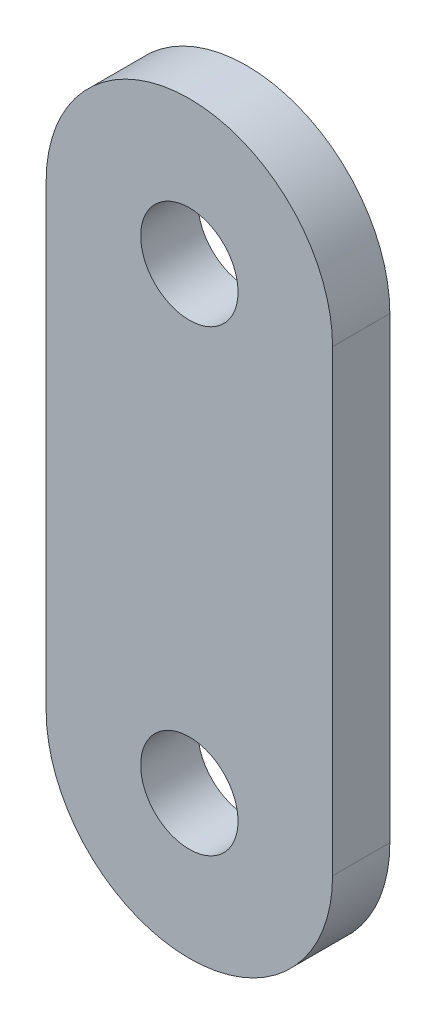
from build123d import *

# Parameters (mm, degrees)
SKETCH1_R           = 8.5
BOSS_EXTRUDE1_DEPTH = 10


with BuildPart() as part:
    # Sketch1 → Boss-Extrude1 (new body)
    with BuildSketch(Plane.XY):
        with BuildLine():
            Line((-25, 0), (-25, 80))
            ThreePointArc((-25, 80), (0, 105), (25, 80))
            Line((25, 80), (25, 0))
            ThreePointArc((25, 0), (0, -25), (-25, 0))
        make_face()
        Circle(SKETCH1_R, mode=Mode.SUBTRACT)
        with Locations((0, 80)):
            Circle(SKETCH1_R, mode=Mode.SUBTRACT)
    extrude(amount=BOSS_EXTRUDE1_DEPTH)


solid = part.part
